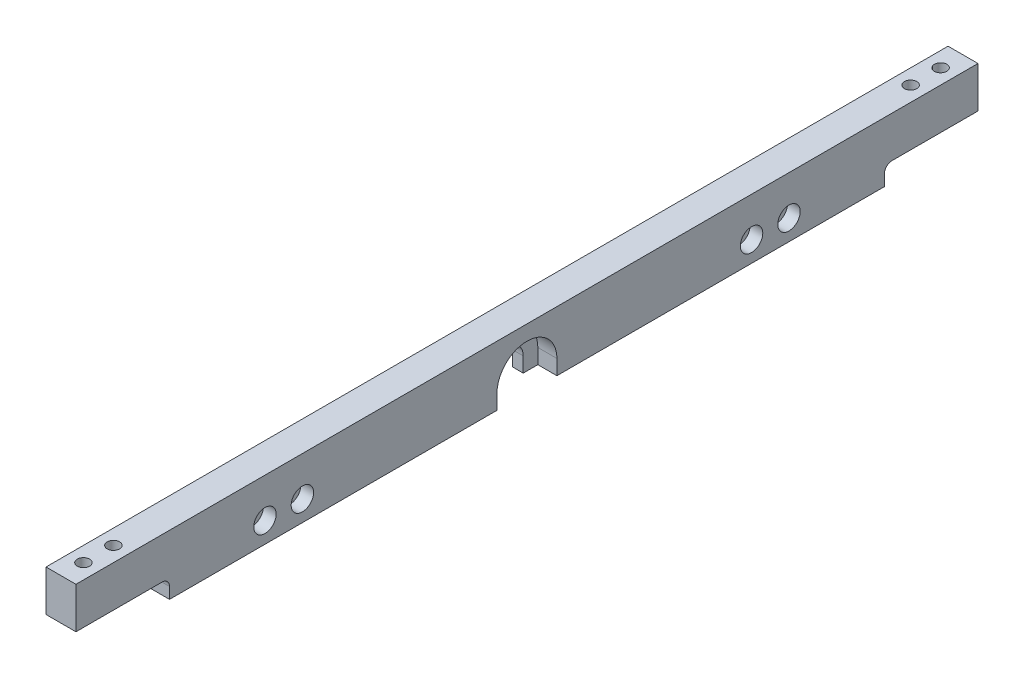
SolidWorks part; units mm, degrees
material "AL6061"
ref_plane "Front Plane" through (0, 0, 0) normal (0, 0, 1) x (1, 0, 0)
ref_plane "Top Plane" through (0, 0, 0) normal (0, 1, 0) x (1, 0, 0)
ref_plane "Right Plane" through (0, 0, 0) normal (1, 0, 0) x (0, 0, -1)
sketch "Sketch3" plane through (0, 0, 0) normal (0, 0, 1) x (1, 0, 0)
  line L0 (0, 0) -> (0, 16)
  line L1 (0, 16) -> (8, 16)
  line L2 (8, 16) -> (8, 0)
  line L5 (8, 0) -> (0, 0)
  dimension "D2" = 8
  dimension "D4" = 16
extrude "Boss-Extrude2" add sketch "Sketch3" along normal blind 241
sketch "Sketch4" plane through (8, 0, 0) normal (1, 0, 0) x (0, 0, -1)
  line L0 (-120.5, 0) -> (-120.5, 16) construction
  line L1 (-241, 0) -> (0, 0) construction
  line L2 (-241, 16) -> (0, 16) construction
  line L3 (-120.5, 4) -> (-120.5, 0) construction
  line L4 (-112.5, 4) -> (-112.5, 0)
  line L5 (-128.5, 4) -> (-128.5, 0)
  arc A0 (-112.5, 4) -> (-128.5, 4) centre (-120.5, 4) ccw
  arc A1 (-128.5, 0) -> (-112.5, 0) centre (-120.5, 0) ccw
  point P7 (-120.5, 2)
  dimension "D1" = 8
  dimension "D2" = 4
extrude "Cut-Extrude1" cut sketch "Sketch4" against normal blind 5.1
sketch "Sketch5" plane through (2.9, 0, 0) normal (1, 0, 0) x (0, 0, -1)
  line L0 (-120.5, 4) -> (-120.5, 0) construction
  line L1 (-128.5, 0) -> (-112.5, 0) construction
  line L2 (-116.4, 4) -> (-116.4, 0)
  line L3 (-124.6, 4) -> (-124.6, 0)
  arc A1 (-116.4, 4) -> (-124.6, 4) centre (-120.5, 4) ccw
  arc A2 (-124.6, 0) -> (-116.4, 0) centre (-120.5, 0) ccw
  point P6 (-120.5, 2)
  dimension "D1" = 4.1
extrude "Cut-Extrude2" cut sketch "Sketch5" against normal through all
hole_wizard "CBORE for M3 Hexagon socket head cap screws1" positions "Sketch6" profile "Sketch7" counterbore size "M3" standard "GB"
sketch "Sketch6" plane through (8, 0, 0) normal (1, 0, 0) x (0, 0, -1)
  line L0 (0, 0) -> (0, 16) construction
  line L1 (-112.5, 0) -> (0, 0) construction
  line L2 (-120.5, 16) -> (-120.5, 0) construction
  line L3 (-241, 16) -> (0, 16) construction
  point P0 (-60.5, 5.5)
  point P2 (-50.5, 5.5)
  point P15 (-190.5, 5.5)
  point P16 (-180.5, 5.5)
  dimension "D1" = 10
  dimension "D2" = 50.5
  dimension "D3" = 5.5
sketch "Sketch7" plane through (8, 5.5, 60.5) normal (0, 1, 0) x (0, 0, -1)
  line L0 (0, 0) -> (0, 11.1215)
  line L1 (0, 11.1215) -> (1.7, 10.1)
  line L2 (1.7, 10.1) -> (1.7, 3.4)
  line L3 (1.7, 3.4) -> (3, 3.4)
  line L4 (3, 3.4) -> (3, 0)
  line L5 (3, 0) -> (0, 0)
  line L10 (0, 11.1215) -> (-1.7, 10.1) construction
  line L11 (0, -6.35) -> (0, 107.95) construction
  dimension "孔直径" = 3.4
  dimension "孔深度" = 10.1
  dimension "柱形沉头孔直径" = 6
  dimension "柱形沉头孔深度" = 3.4
  dimension "导头角度" = 118
hole_wizard "M4 Tapped Hole1" positions "Sketch8" profile "Sketch9" tap size "M4" standard "GB"
sketch "Sketch8" plane through (0, 16, 0) normal (0, 1, 0) x (1, 0, 0)
  line L6 (0, -241) -> (0, 0) construction
  line L9 (8, -120.5) -> (0, -120.5) construction
  line L10 (8, -241) -> (8, 0) construction
  point P15 (4, -235)
  point P24 (4, -227)
  point P36 (4, -14)
  point P37 (4, -6)
  dimension "D1" = 4
  dimension "D2" = 106.5
  dimension "D3" = 8
sketch "Sketch9" plane through (4, 16, 235) normal (1, 0, 0) x (0, 0, 1)
  line L0 (0, 0) -> (0, 10.0914)
  line L1 (0, 10.0914) -> (1.65, 9.1)
  line L2 (1.65, 9.1) -> (1.65, 0)
  line L5 (1.65, 0) -> (0, 0)
  line L10 (0, 10.0914) -> (-1.65, 9.1) construction
  line L11 (0, -6.35) -> (0, 107.95) construction
  dimension "螺纹孔钻头直径" = 3.3
  dimension "螺纹孔钻头深度" = 9.1
  dimension "导头角度" = 118
cosmetic thread "Cosmetic Thread 1" parameters "D1"=7, "D2"=4
cosmetic thread "Cosmetic Thread 2" parameters "D1"=7, "D2"=4
cosmetic thread "Cosmetic Thread 3" parameters "D1"=7, "D2"=4
cosmetic thread "Cosmetic Thread 4" parameters "D1"=7, "D2"=4
sketch "Sketch10" plane through (8, 0, 0) normal (1, 0, 0) x (0, 0, -1)
  line L0 (-120.5, 16) -> (-120.5, 4) construction
  line L1 (0, 0) -> (-25, 0)
  line L2 (0, 0) -> (0, 5)
  line L3 (0, 5) -> (-23, 5)
  line L4 (-25, 0) -> (-25, 3)
  line L5 (-241, 16) -> (0, 16) construction
  line L6 (-216, 0) -> (-216, 3)
  line L7 (-241, 5) -> (-218, 5)
  line L8 (-241, 0) -> (-241, 5)
  line L9 (-241, 0) -> (-216, 0)
  arc A0 (-23, 5) -> (-25, 3) centre (-23, 3) ccw
  arc A1 (-218, 5) -> (-216, 3) centre (-218, 3) cw
  dimension "D3" = 2
  dimension "D1" = 5
  dimension "D2" = 25
extrude "Cut-Extrude3" cut sketch "Sketch10" against normal through all
